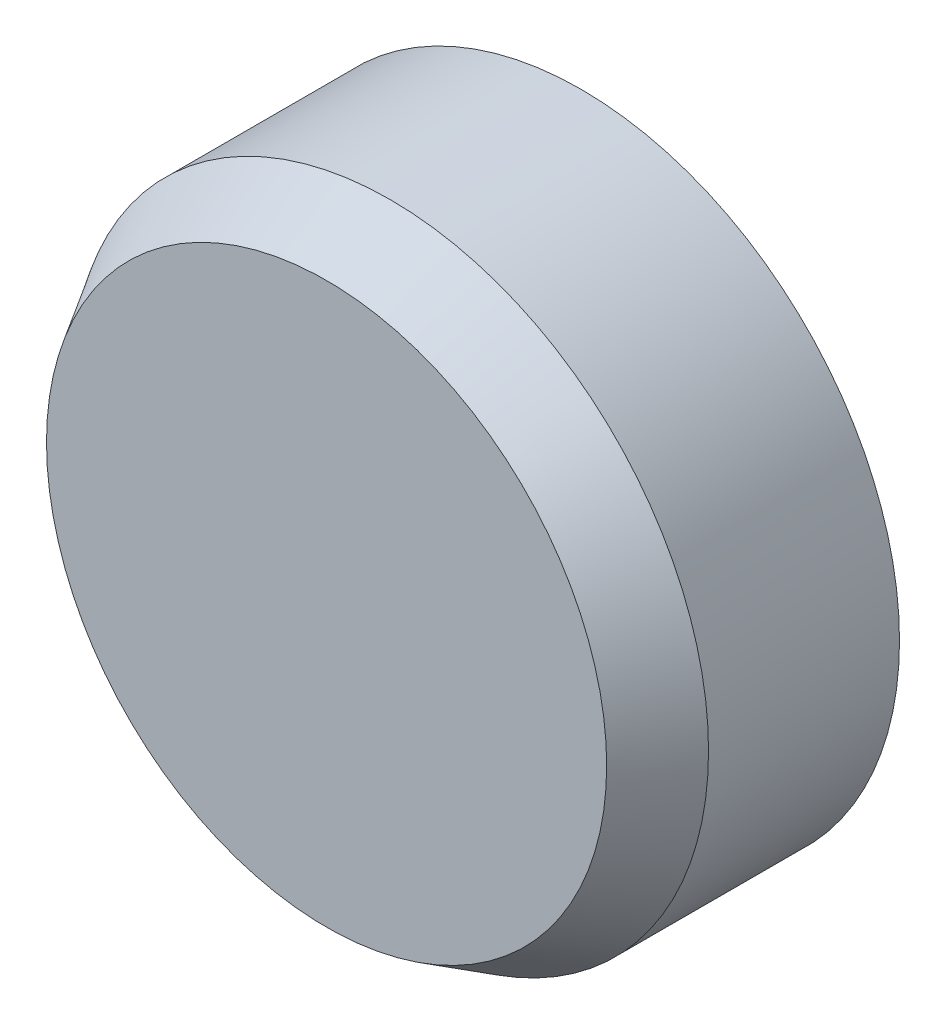
from build123d import *

# Parameters (mm, degrees)
SKETCH1_R             = 50
BOSS_EXTRUDE1_DEPTH   = 40
CHAMFER1_SIZE         = 10
CHAMFER1_SIZE2        = 6
M6_TAPPED_HOLE1_D     = 5
M6_TAPPED_HOLE1_DEPTH = 17
M6_TAPPED_HOLE1_TIP   = 1.502151548


with BuildPart() as part:
    # Sketch1 → Boss-Extrude1 (new body)
    with BuildSketch(Plane.XY):
        Circle(SKETCH1_R)
    extrude(amount=BOSS_EXTRUDE1_DEPTH)

    # Chamfer1
    chamfer1_edges = [part.edges().sort_by_distance(p)[0] for p in [
        (-50, 0, 40),
    ]]
    chamfer1_side = [part.faces().sort_by_distance(p)[0] for p in [
        (-50, 0, 20),
    ]]
    chamfer(chamfer1_edges, length=CHAMFER1_SIZE, length2=CHAMFER1_SIZE2, reference=chamfer1_side[0])

    # M6 Tapped Hole1
    with Locations(Plane(origin=(0, 0, 0), x_dir=(-1, 0, 0), z_dir=(0, 0, -1))):
        with Locations((0, 0)):
            Hole(M6_TAPPED_HOLE1_D / 2, depth=M6_TAPPED_HOLE1_DEPTH)
            with Locations((0, 0, -(M6_TAPPED_HOLE1_DEPTH + M6_TAPPED_HOLE1_TIP / 2))):  # 118° drill point
                Cone(0, M6_TAPPED_HOLE1_D / 2, M6_TAPPED_HOLE1_TIP, mode=Mode.SUBTRACT)


solid = part.part
